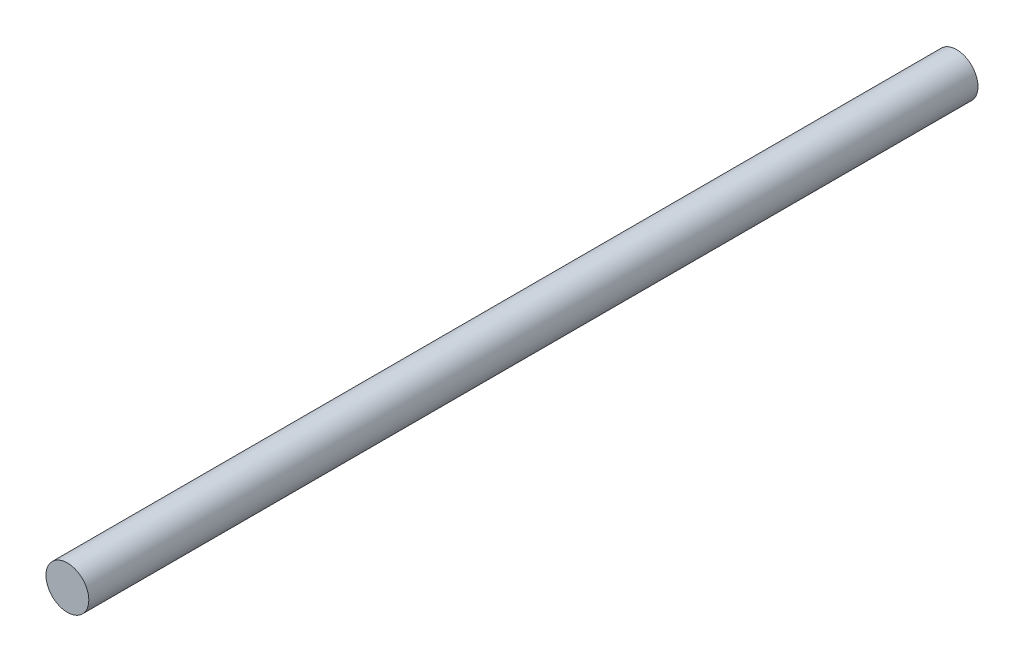
from build123d import *

# Parameters (mm, degrees)
SKETCH1_R           = 6
BOSS_EXTRUDE1_DEPTH = 124.5


with BuildPart() as part:
    # Sketch1 → Boss-Extrude1 (new, symmetric)
    with BuildSketch(Plane.XY):
        Circle(SKETCH1_R)
    extrude(amount=BOSS_EXTRUDE1_DEPTH, both=True)


solid = part.part
